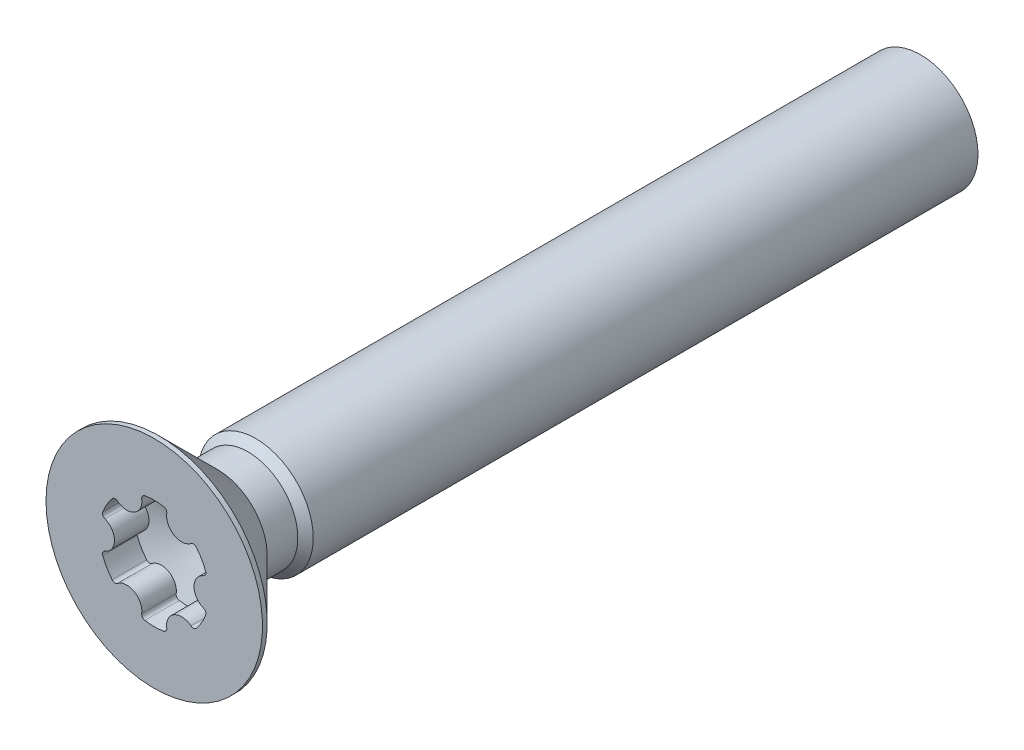
from build123d import *

# Parameters (mm, degrees)
SKETCH1_R          = 3
BASE_EXTRUDE_DEPTH = 34.7
CUT_EXTRUDE1_DEPTH = 1.8


with BuildPart() as part:
    # Sketch1 → Base-Extrude (new body)
    with BuildSketch(Plane.XY):
        Circle(SKETCH1_R)
    extrude(amount=BASE_EXTRUDE_DEPTH)

    # Sketch6 → Base-Revolve2 (revolve)
    with BuildSketch(Plane(origin=(0, 0, 0), x_dir=(1, 0, 0), z_dir=(0, 1, 0)), mode=Mode.PRIVATE) as base_revolve2_sk:
        Polygon((2.598, -36.7), (5.65, -39.752), (5.65, -40), (0, -40), (0, -34.7), (3, -34.7), (2.598, -35.102), align=None)
    revolve(base_revolve2_sk.sketch.rotate(Axis((0, 0, -0.393620135), (0, 0, 1)), 180), axis=Axis((0, 0, -0.393620135), (0, 0, 1)))

    # Sketch7 → Cut-Extrude1 (cut)
    with BuildSketch(Plane.XY.offset(40)):
        with BuildLine():
            ThreePointArc((0.489815827, 2.817743859), (0, 2.86), (-0.489815827, 2.817743859))
            ThreePointArc((-0.489815827, 2.817743859), (-0.617632508, 2.737888703), (-0.653418206, 2.591487427))
            ThreePointArc((-0.653418206, 2.591487427), (-1.0375, 1.797002713), (-1.917584843, 1.861620479))
            ThreePointArc((-1.917584843, 1.861620479), (-2.062264916, 1.903829794), (-2.19532985, 1.833064879))
            ThreePointArc((-2.19532985, 1.833064879), (-2.476832655, 1.43), (-2.685145677, 0.984678981))
            ThreePointArc((-2.685145677, 0.984678981), (-2.679897424, 0.83405891), (-2.571003048, 0.729866948))
            ThreePointArc((-2.571003048, 0.729866948), (-2.075, 0), (-2.571003048, -0.729866948))
            ThreePointArc((-2.571003048, -0.729866948), (-2.679897424, -0.83405891), (-2.685145677, -0.984678981))
            ThreePointArc((-2.685145677, -0.984678981), (-2.476832655, -1.43), (-2.19532985, -1.833064879))
            ThreePointArc((-2.19532985, -1.833064879), (-2.062264916, -1.903829794), (-1.917584843, -1.861620479))
            ThreePointArc((-1.917584843, -1.861620479), (-1.0375, -1.797002713), (-0.653418206, -2.591487427))
            ThreePointArc((-0.653418206, -2.591487427), (-0.617632508, -2.737888703), (-0.489815827, -2.817743859))
            ThreePointArc((-0.489815827, -2.817743859), (0, -2.86), (0.489815827, -2.817743859))
            ThreePointArc((0.489815827, -2.817743859), (0.617632508, -2.737888703), (0.653418206, -2.591487427))
            ThreePointArc((0.653418206, -2.591487427), (1.0375, -1.797002713), (1.917584843, -1.861620479))
            ThreePointArc((1.917584843, -1.861620479), (2.062264916, -1.903829794), (2.19532985, -1.833064879))
            ThreePointArc((2.19532985, -1.833064879), (2.476832655, -1.43), (2.685145677, -0.984678981))
            ThreePointArc((2.685145677, -0.984678981), (2.679897424, -0.83405891), (2.571003048, -0.729866948))
            ThreePointArc((2.571003048, -0.729866948), (2.075, 0), (2.571003048, 0.729866948))
            ThreePointArc((2.571003048, 0.729866948), (2.679897424, 0.83405891), (2.685145677, 0.984678981))
            ThreePointArc((2.685145677, 0.984678981), (2.476832655, 1.43), (2.19532985, 1.833064879))
            ThreePointArc((2.19532985, 1.833064879), (2.062264916, 1.903829794), (1.917584843, 1.861620479))
            ThreePointArc((1.917584843, 1.861620479), (1.0375, 1.797002713), (0.653418206, 2.591487427))
            ThreePointArc((0.653418206, 2.591487427), (0.617632508, 2.737888703), (0.489815827, 2.817743859))
        make_face()
    extrude(amount=-CUT_EXTRUDE1_DEPTH, mode=Mode.SUBTRACT)

    # Sketch8 → 切除－旋转1 (revolve, cut)
    with BuildSketch(Plane(origin=(0, 0, 0), x_dir=(1, 0, 0), z_dir=(0, 1, 0))):
        Polygon((0, -38.2), (2.86, -38.2), (0, -37.15904513), align=None)
    revolve(axis=Axis((0, 0, 0), (0, 0, 1)), mode=Mode.SUBTRACT)


solid = part.part
